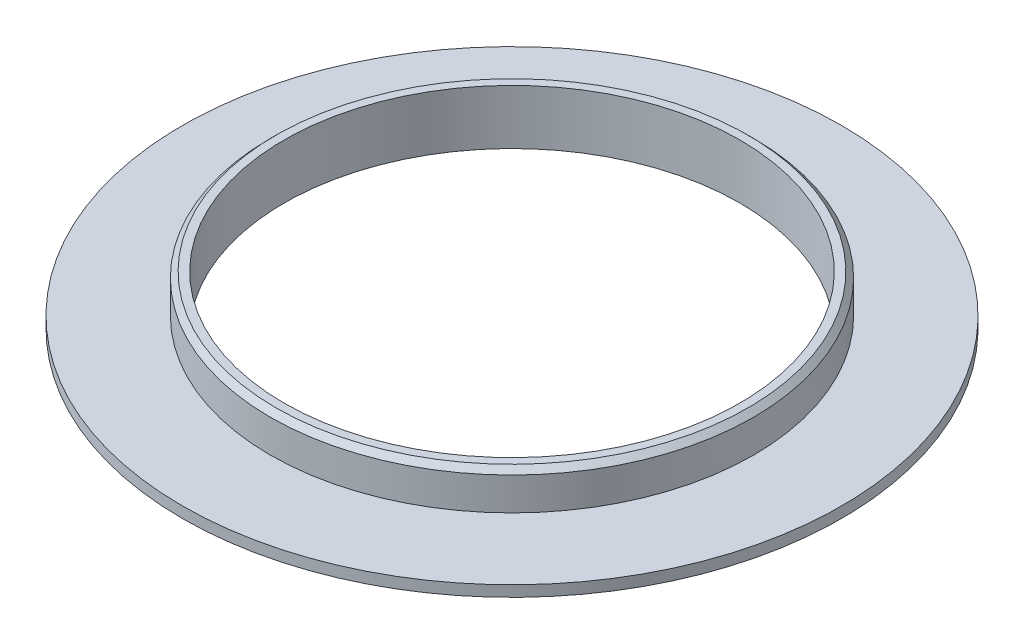
from build123d import *

# Parameters (mm, degrees)
SKETCH_1_R          = 30.147889755
SKETCH_1_R_2        = 20.85
EXTRUDE_1_DEPTH     = 1.5
SKETCH_2_R          = 22.1
SKETCH_2_R_2        = 20.85
EXTRUDE_2_DEPTH     = 3.5
CHAMFER_C0_5_1_SIZE = 0.5
CHAMFER_2_SIZE      = 0.5
CHAMFER_2_SIZE2     = 1.866025404


with BuildPart() as part:
    # 草图1 → 凸台-拉伸1 (new body)
    with BuildSketch(Plane(origin=(0, 0, 0), x_dir=(1, 0, 0), z_dir=(0, 1, 0))):
        with Locations(Location((0, 0, 0), (0, 0, 270))):
            Circle(SKETCH_1_R)
        with Locations(Location((0, 0, 0), (0, 0, 270))):
            Circle(SKETCH_1_R_2, mode=Mode.SUBTRACT)
    extrude(amount=EXTRUDE_1_DEPTH)

    # 草图2 → 凸台-拉伸2 (add)
    with BuildSketch(Plane(origin=(0, 1.5, 0), x_dir=(1, 0, 0), z_dir=(0, 1, 0))):
        with Locations(Location((0, 0, 0), (0, 0, 270))):
            Circle(SKETCH_2_R)
        with Locations(Location((0, 0, 0), (0, 0, 270))):
            Circle(SKETCH_2_R_2, mode=Mode.SUBTRACT)
    extrude(amount=EXTRUDE_2_DEPTH)

    # C0.5 倒角1
    chamfer_c0_5_1_edges = [part.edges().sort_by_distance(p)[0] for p in [
        (0, 5, -22.1),
    ]]
    chamfer(chamfer_c0_5_1_edges, length=CHAMFER_C0_5_1_SIZE)

    # 倒角2
    chamfer_2_edges = [part.edges().sort_by_distance(p)[0] for p in [
        (0, 0, -30.147889755),
    ]]
    chamfer_2_side = [part.faces().sort_by_distance(p)[0] for p in [
        (0, 0.75, -30.147889755),
    ]]
    chamfer(chamfer_2_edges, length=CHAMFER_2_SIZE, length2=CHAMFER_2_SIZE2, reference=chamfer_2_side[0])


solid = part.part
